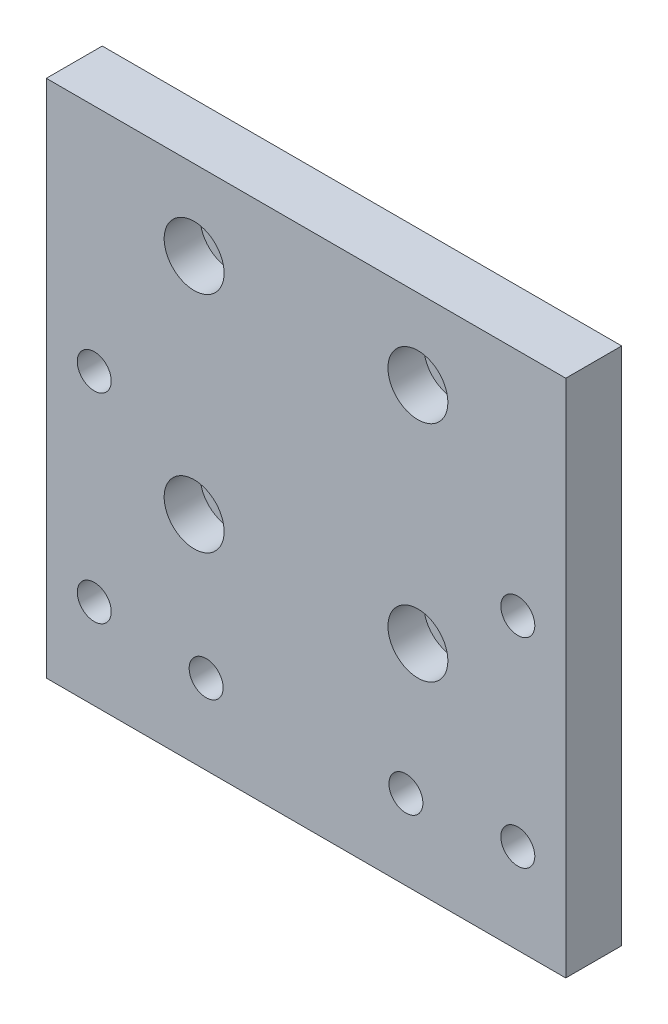
SolidWorks part; units mm, degrees
material "普通碳钢"
ref_plane "Front Plane" through (0, 0, 0) normal (0, 0, 1) x (1, 0, 0)
ref_plane "Top Plane" through (0, 0, 0) normal (0, 1, 0) x (1, 0, 0)
ref_plane "Right Plane" through (0, 0, 0) normal (1, 0, 0) x (0, 0, -1)
sketch "Sketch1" plane through (0, 0, 0) normal (0, 0, 1) x (1, 0, 0)
  line L1 (0, 0) -> (130, 0)
  line L2 (0, 0) -> (0, 130)
  line L3 (0, 130) -> (130, 130)
  line L4 (130, 0) -> (130, 130)
  dimension "D1" = 130
  dimension "D2" = 130
extrude "Boss-Extrude1" add sketch "Sketch1" along normal blind 14
hole_wizard "Hole Size (%based on) Socket Head Cap Screw Type1" positions "Sketch3" profile "Sketch4" counterbore size "M8" standard "GB" end condition through all
sketch "Sketch3" plane through (0, 0, 14) normal (0, 0, 1) x (1, 0, 0)
  line L0 (37, 110) -> (93, 110) construction
  line L1 (93, 110) -> (93, 54) construction
  line L2 (93, 54) -> (37, 54) construction
  line L3 (37, 54) -> (37, 110) construction
  line L5 (65, 110) -> (65, 130) construction
  line L6 (130, 130) -> (0, 130) construction
  point P0 (37, 110)
  point P2 (93, 110)
  point P4 (93, 54)
  point P6 (37, 54)
  dimension "D1" = 56
  dimension "D2" = 56
  dimension "D3" = 20
sketch "Sketch4" plane through (37, 110, 14) normal (1, 0, 0) x (0, -1, 0)
  line L0 (0, 0) -> (0, 14)
  line L1 (0, 14) -> (4.5, 14)
  line L3 (4.5, 14) -> (4.5, 9)
  line L4 (4.5, 9) -> (7.5, 9)
  line L5 (7.5, 9) -> (7.5, 0)
  line L7 (7.5, 0) -> (0, 0)
  line L11 (0, -6.35) -> (0, 107.95) construction
  dimension "通孔孔直径" = 9
  dimension "通孔孔深度" = 14
  dimension "柱形沉头孔直径" = 15
  dimension "柱形沉头孔深度" = 9
hole_wizard "M10 Tapped Hole1" positions "Sketch5" profile "Sketch6" tap size "M10" standard "GB" end condition through all
sketch "Sketch5" plane through (0, 0, 0) normal (0, 0, -1) x (-1, 0, 0)
  line L0 (-90, 20) -> (-40, 20) construction
  line L2 (-65, 20) -> (-65, 0) construction
  line L3 (0, 0) -> (-130, 0) construction
  point P0 (-90, 20)
  point P2 (-40, 20)
  dimension "D1" = 20
  dimension "D2" = 50
sketch "Sketch6" plane through (90, 20, 0) normal (1, 0, 0) x (0, 1, 0)
  line L0 (0, 0) -> (0, 14)
  line L1 (0, 14) -> (4.25, 14)
  line L2 (4.25, 14) -> (4.25, 0)
  line L5 (4.25, 0) -> (0, 0)
  line L11 (0, -6.35) -> (0, 107.95) construction
  dimension "通孔螺纹孔钻头直径" = 8.5
  dimension "通孔螺纹孔钻头深度" = 14
cosmetic thread "Hole Thread Line1" parameters "D2"=10
cosmetic thread "Hole Thread Line2" parameters "D2"=10
sketch "Sketch7" plane through (0, 130, 0) normal (0, 1, 0) x (1, 0, 0)
  line L4 (130, 0) -> (0, 0)
  line L5 (0, 0) -> (0, -14)
  line L6 (0, -14) -> (130, -14)
  line L7 (130, -14) -> (130, 0)
  line L8 (130, 0) -> (0, 0)
  line L9 (0, 0) -> (0, -14)
  line L10 (0, -14) -> (130, -14)
  line L11 (130, -14) -> (130, 0)
  dimension "D1" = 0
extrude "Boss-Extrude2" [suppressed] add sketch "Sketch7" along normal blind 20
hole_wizard "M10 Tapped Hole2" positions "Sketch8" profile "Sketch9" tap size "M10" standard "GB" end condition through all
sketch "Sketch8" plane through (0, 0, 0) normal (0, 0, -1) x (-1, 0, 0)
  line L0 (0, 0) -> (-130, 0) construction
  line L1 (-130, 0) -> (-130, 130) construction
  line L2 (0, 130) -> (0, 0) construction
  point P0 (-118, 72.5)
  point P2 (-118, 22.5)
  point P4 (-12, 72.5)
  point P6 (-12, 22.5)
  dimension "D1" = 22.5
  dimension "D2" = 50
  dimension "D3" = 12
  dimension "D4" = 12
sketch "Sketch9" plane through (118, 72.5, 0) normal (1, 0, 0) x (0, 1, 0)
  line L0 (0, 0) -> (0, 14)
  line L1 (0, 14) -> (4.25, 14)
  line L2 (4.25, 14) -> (4.25, 0)
  line L5 (4.25, 0) -> (0, 0)
  line L11 (0, -6.35) -> (0, 107.95) construction
  dimension "通孔螺纹孔钻头直径" = 8.5
  dimension "通孔螺纹孔钻头深度" = 14
cosmetic thread "Hole Thread Line3" parameters "D2"=10
cosmetic thread "Hole Thread Line4" parameters "D2"=10
cosmetic thread "Hole Thread Line5" parameters "D2"=10
cosmetic thread "Hole Thread Line6" parameters "D2"=10
